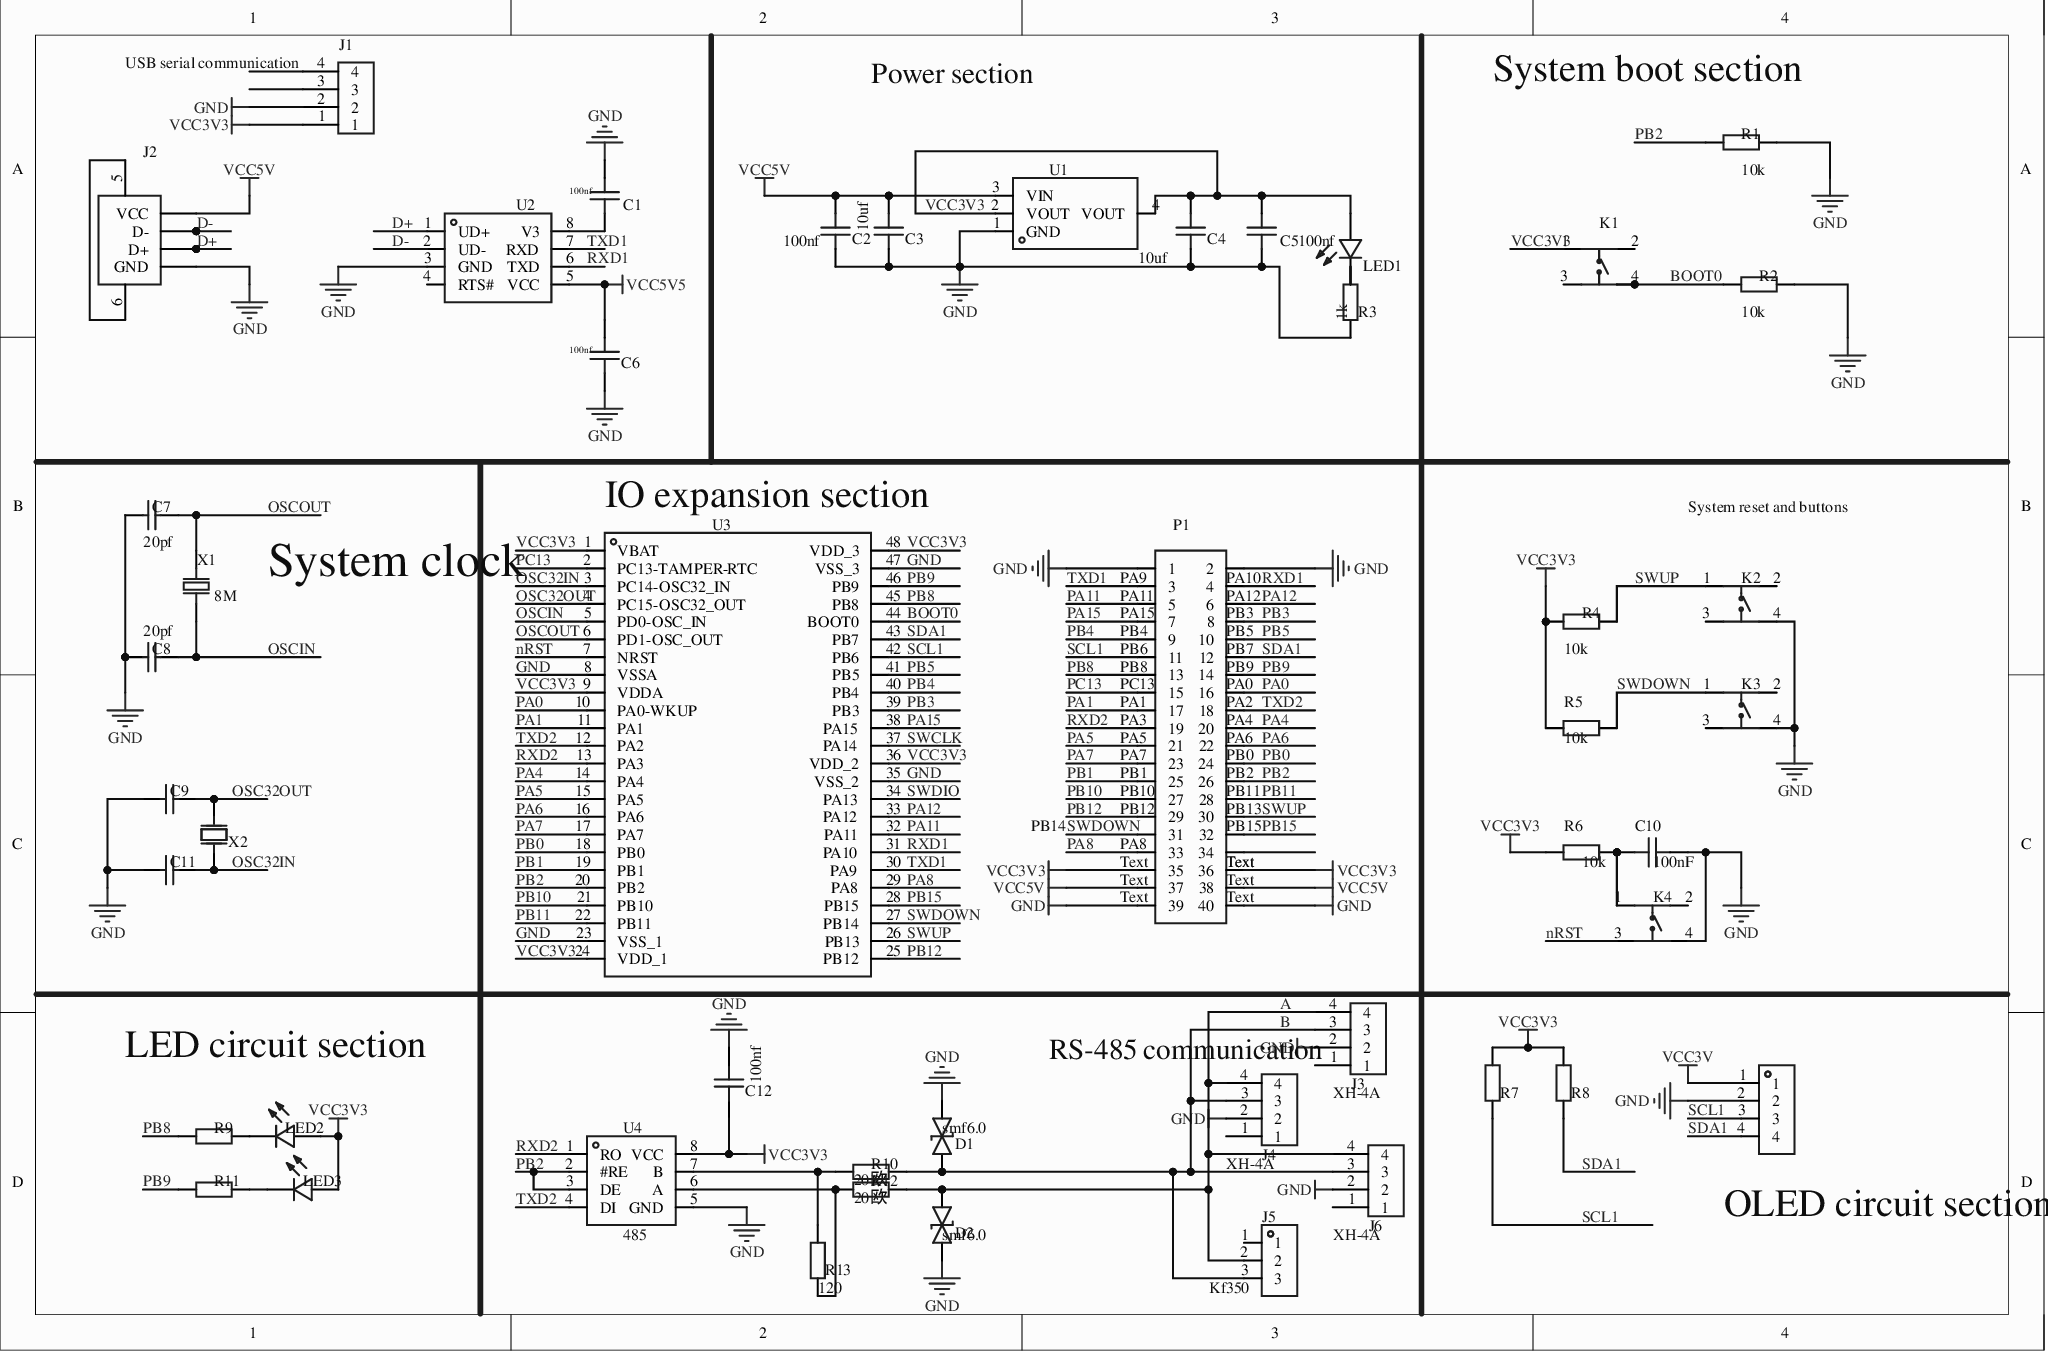
[diagram p0: MISC51869-3.schdoc]
# Altium project MISC51869-2.PrjPcb
1 sheet, 48 parts. Net scope: global (net labels, ports and power ports of the same name join across sheets).
Board file: MISC51869.pcbdoc

## Sheet MISC51869-3.schdoc
size 292 x 193 mm; SheetNumber: 1; SheetTotal: 1; Name: MISC51869

### Parts
C1  CC0603KRX7R9BB104  [C0603 - duplicate]  (value not drawn)
C2  CL21A106KAYNNNE  [C0805]  (value not drawn)
C3  CC0603KRX7R9BB104  [C0603 - duplicate]  (value not drawn)
C4  CL21A106KAYNNNE  [C0805]  (value not drawn)
C5  CC0603KRX7R9BB104  [C0603 - duplicate]  (value not drawn)
C6  CC0603KRX7R9BB104  [C0603 - duplicate]  (value not drawn)
C7  CL10C200JB8NNNC  [C0603c20pf]  (value not drawn)
C8  CL10C200JB8NNNC  [C0603c20pf]  (value not drawn)
C9  CL10C200JB8NNNC  [C0603c20pf]  (value not drawn)
C10  CL21A106KAYNNNE  [C0805]  (value not drawn)
C11  CL10C200JB8NNNC  [C0603c20pf]  (value not drawn)
C12  CC0603KRX7R9BB104  [C0603 - duplicate]  (value not drawn)
D1  SMF6.0CA_C2990473  [瞬态二极管]  (value not drawn)
D2  SMF6.0CA_C2990473  [瞬态二极管]  (value not drawn)
H1  PM254V-11-04-H85  [排母4p]  (value not drawn)
J1  XH-4A  [XH-4A]  (value not drawn)
J2  USB-B-Female-90  [USB-B_TH_USB-B-FEMALE-90]  (value not drawn)
J3  XH-4A  [XH-4A]  (value not drawn)
J4  XH-4A  [XH-4A]  (value not drawn)
J5  KF350-3.5-3P  [KF350-3.5-3P]  (value not drawn)
J6  XH-4A  [XH-4A]  (value not drawn)
K1  KH-6X6X5H-STM  [按键]  (value not drawn)
K2  KH-6X6X5H-STM  [复位按键]  (value not drawn)
K3  KH-6X6X5H-STM  [复位按键]  (value not drawn)
K4  KH-6X6X5H-STM  [复位按键]  (value not drawn)
LED1  FC-D1608HGK-572C  [LED0603-RD]  (value not drawn)
LED2  FC-D1608HGK-572C  [LED0603-RD]  (value not drawn)
LED3  FC-D1608HGK-572C  [LED0603-RD]  (value not drawn)
P1  Header-Male-2.54_2x20  [HDR-TH_40P-P2.54-V-M-R2-C20-S2.54]  (value not drawn)
R1  0603WAF1002T5E  [电阻R0603]  (value not drawn)
R2  0603WAF1002T5E  [电阻R0603]  (value not drawn)
R3  0603WAF1001T5E  [C0603 - duplicate]  (value not drawn)
R4  0603WAF1002T5E  [电阻R0603]  (value not drawn)
R5  0603WAF1002T5E  [电阻R0603]  (value not drawn)
R6  0603WAF1002T5E  [电阻R0603]  (value not drawn)
R7  0603WAF4701T5E  [R06034.7k]  (value not drawn)
R8  0603WAF4701T5E  [R06034.7k]  (value not drawn)
R9  0603WAF1001T5E  [R06031k]  (value not drawn)
R10  0805W8F200JT5E  [R0805]  (value not drawn)
R11  0603WAF1001T5E  [R06031k]  (value not drawn)
R12  0805W8F200JT5E  [R0805]  (value not drawn)
R13  0603WAF1200T5E  [R0603 - duplicate]  (value not drawn)
U1  AMS1117-3.3  [SOT-223-3_L6.5-W3.4-P2.30-LS7.0-BR]  (value not drawn)
U2  CH340N_C2977777  [SOP-8_L4.9-W3.9-P1.27-LS6.0-BL]  (value not drawn)
U3  STM32F103C8T6  [LQFP-48_L7.0-W7.0-P0.50-LS9.0-BL]  (value not drawn)
U4  SP3485EEN  [485SOP-8_L5.0-W4.0-P1.27-LS6.0-BL]  (value not drawn)
X1  Q13FC1350000400  [CRYSTAL-SMD_L5.0-W3.2]  (value not drawn)
X2  X50328MSB2GI  [FC-135R_L3.2-W1.5]  (value not drawn)

### Nets
GND: C1.2 C2.1 C3.2 C4.1 C5.1 C6.1 C7.1 C8.1 C9.1 C10.1 C11.1 C12.2 D1.2 D2.1 H1.2 J1.2 J2.4(GND) J3.2 J4.2 J6.2 K2.4 K3.4 K4.4 P1.1 P1.2 P1.39 P1.40 R1.2 R2.2 R3.1 U1.1(GND) U2.3(GND) U3.8(VSSA) U3.23(VSS_1) U3.35(VSS_2) U3.47(VSS_3) U4.5(GND)
VCC3V: H1.1
VCC3V3: C4.2 C5.2 C12.1 J1.1 K1.1 LED1.2(+) LED2.2(+) LED3.2(+) P1.35 P1.36 R4.1 R5.1 R6.1 R7.2 R8.2 U1.2(VOUT) U1.4(VOUT) U3.1(VBAT) U3.9(VDDA) U3.24(VDD_1) U3.36(VDD_2) U3.48(VDD_3) U4.8(VCC)
VCC5V: C2.2 C3.1 J2.1(VCC) P1.37 P1.38 U1.3(VIN)
VCC5V5: C6.2 U2.5(VCC)
A: D2.2 J3.4 J4.4 J5.2 J6.4 R12.2
B: D1.1 J3.3 J4.3 J5.3 J6.3 R10.2
BOOT0: K1.4 R2.1 U3.44(BOOT0)
D+: J2.3(D+) U2.1(UD+)
D-: J2.2(D-) U2.2(UD-)
nRST: K4.3 U3.7(NRST)
OSC32IN: C11.2 U3.3(PC14-OSC32_IN) X2.2(OSC2)
OSC32OUT: C9.2 U3.4(PC15-OSC32_OUT) X2.1(OSC1)
OSCIN: C8.2 U3.5(PD0-OSC_IN) X1.2
OSCOUT: C7.2 U3.6(PD1-OSC_OUT) X1.1
PA0: P1.16 U3.10(PA0-WKUP)
PA1: P1.17 U3.11(PA1)
PA4: P1.20 U3.14(PA4)
PA5: P1.21 U3.15(PA5)
PA6: P1.22 U3.16(PA6)
PA7: P1.23 U3.17(PA7)
PA8: P1.33 U3.29(PA8)
PA11: P1.5 U3.32(PA11)
PA12: P1.6 U3.33(PA12)
PA15: P1.7 U3.38(PA15)
PB0: P1.24 U3.18(PB0)
PB1: P1.25 U3.19(PB1)
PB2: P1.26 R1.1 U3.20(PB2) U4.2(#RE) U4.3(DE)
PB3: P1.8 U3.39(PB3)
PB4: P1.9 U3.40(PB4)
PB5: P1.10 U3.41(PB5)
PB8: P1.13 R9.1 U3.45(PB8)
PB9: P1.14 R11.1 U3.46(PB9)
PB10: P1.27 U3.21(PB10)
PB11: P1.28 U3.22(PB11)
PB12: P1.29 U3.25(PB12)
PB15: P1.32 U3.28(PB15)
PC13: P1.15 U3.2(PC13-TAMPER-RTC)
RXD1: P1.4 U2.6(TXD) U3.31(PA10)
RXD2: P1.19 U3.13(PA3) U4.1(RO)
SCL1: H1.3 P1.11 R7.1 U3.42(PB6)
SDA1: H1.4 P1.12 R8.1 U3.43(PB7)
SWCLK: U3.37(PA14)
SWDIO: U3.34(PA13)
SWDOWN: K3.1 P1.31 R5.2 U3.27(PB14)
SWUP: K2.1 P1.30 R4.2 U3.26(PB13)
TXD1: P1.3 U2.7(RXD) U3.30(PA9)
TXD2: P1.18 U3.12(PA2) U4.4(DI)
NetC1_1: C1.1 U2.8(V3)
NetC10_2: C10.2 K4.1 R6.2
NetJ2_5: J2.5(SH1) J2.6(SH2)
NetLED1_1: LED1.1(-) R3.2
NetLED2_1: LED2.1(-) R9.2
NetLED3_1: LED3.1(-) R11.2
NetR10_1: R10.1 R13.2 U4.7(B)
NetR12_1: R12.1 R13.1 U4.6(A)

Not connected (* = marked no-connect by the designer): J1 3* 4*; J3 1; J4 1; J5 1; J6 1; K1 2 3; K2 2 3; K3 2 3; K4 2; P1 34; U2 4(RTS#)

### Notes on the sheet
- (near J1) USB serial communication
- Power section
- (near R1) System boot section
- (near C1) 100nf
- 10uf
- (near R1) 10k
- (near C2) 100nf
- (near LED1) 100nf
- (near R3) 1k
- (near R2) 10k
- (near C6) 100nf
- 20pf
- System clock
- (near U3) IO expansion section
- (near P1) PA9
- (near P1) PA10
- System reset and buttons
- (near X1) 8M
- (near P1) PA11
- (near P1) PA15
- (near P1) PB4
- (near P1) PB6
- (near P1) PB8
- (near P1) PA12
- (near P1) PB3
- (near P1) PB5
- (near P1) PB7
- (near P1) PB9
- (near R4) 10k
- (near P1) PC13
- (near P1) PA1
- (near P1) PA3
- (near P1) PA5
- (near P1) PA7
- (near P1) PA0
- (near P1) PA2
- (near P1) PA4
- (near P1) PA6
- (near P1) PB0
- (near R5) 10k
- PB14
- (near P1) PB1
- (near P1) PB10
- (near P1) PB12
- (near P1) PA8
- (near P1) PB2
- (near P1) PB11
- (near P1) PB13
- (near P1) PB15
- (near P1) Text
- (near R6) 10k
- (near C10) 100nF
- LED circuit section
- (near C12) 100nf
- RS-485 communication
- (near J3) XH-4A
- (near R12) 20欧
- 20欧
- (near D1) smf6.0
- (near J4) XH-4A
- (near U4) 485
- (near R13) 120
- (near D2) smf6.0
- (near J5) Kf350
- (near J6) XH-4A
- (near H1) OLED circuit section

### Library data of the parts
C1 = CC0603KRX7R9BB104: OriginFootprint 2: C0603; UniqueId: 5fb4f22ffcb6a001; AddInBom: yes; Device: CC0603KRX7R9BB104; DesignItemID: CC0603KRX7R9BB104; SymbolName: CC0603KRX7R9BB104; FootprintName: C0603 - duplicate
C2 = CL21A106KAYNNNE: UniqueId: 21d50210554cb61f; AddInBom: yes; Device: CL21A106KAYNNNE; DesignItemID: CL21A106KAYNNNE; SymbolName: CL21A106KAYNNNE; FootprintName: C0805
C3 = CC0603KRX7R9BB104: OriginFootprint 2: C0603; UniqueId: ec64484c8c07847f; AddInBom: yes; Device: CC0603KRX7R9BB104; DesignItemID: CC0603KRX7R9BB104; SymbolName: CC0603KRX7R9BB104; FootprintName: C0603 - duplicate
C4 = CL21A106KAYNNNE: UniqueId: 623e2bb2442f04df; AddInBom: yes; Device: CL21A106KAYNNNE; DesignItemID: CL21A106KAYNNNE; SymbolName: CL21A106KAYNNNE; FootprintName: C0805
C5 = CC0603KRX7R9BB104: OriginFootprint 2: C0603; UniqueId: 05d417a4d81547fc; AddInBom: yes; Device: CC0603KRX7R9BB104; DesignItemID: CC0603KRX7R9BB104; SymbolName: CC0603KRX7R9BB104; FootprintName: C0603 - duplicate
C6 = CC0603KRX7R9BB104: OriginFootprint 2: C0603; UniqueId: d45ffe04e43665a4; AddInBom: yes; Device: CC0603KRX7R9BB104; DesignItemID: CC0603KRX7R9BB104; SymbolName: CC0603KRX7R9BB104; FootprintName: C0603 - duplicate
C7 = CL10C200JB8NNNC: UniqueId: 3007ca2539a35480; AddInBom: yes; Device: CL10C200JB8NNNC; DesignItemID: CL10C200JB8NNNC; SymbolName: CL10C200JB8NNNC; FootprintName: C0603c20pf
C8 = CL10C200JB8NNNC: UniqueId: 878ab3ab0cce2757; AddInBom: yes; Device: CL10C200JB8NNNC; DesignItemID: CL10C200JB8NNNC; SymbolName: CL10C200JB8NNNC; FootprintName: C0603c20pf
C9 = CL10C200JB8NNNC: UniqueId: 60e6893b044e2f17; AddInBom: yes; Device: CL10C200JB8NNNC; DesignItemID: CL10C200JB8NNNC; SymbolName: CL10C200JB8NNNC; FootprintName: C0603c20pf
C10 = CL21A106KAYNNNE: UniqueId: c1764753ee6525b4; AddInBom: yes; Device: CL21A106KAYNNNE; DesignItemID: CL21A106KAYNNNE; SymbolName: CL21A106KAYNNNE; FootprintName: C0805
C11 = CL10C200JB8NNNC: UniqueId: b49c3108c5288e9f; AddInBom: yes; Device: CL10C200JB8NNNC; DesignItemID: CL10C200JB8NNNC; SymbolName: CL10C200JB8NNNC; FootprintName: C0603c20pf
C12 = CC0603KRX7R9BB104: UniqueId: 4eba2014d94c20ef; OriginFootprint 2: C0603; AddInBom: yes; Device: CC0603KRX7R9BB104; DesignItemID: CC0603KRX7R9BB104; SymbolName: CC0603KRX7R9BB104; FootprintName: C0603 - duplicate
D1 = SMF6.0CA_C2990473: UniqueId: 07a0d5848cd81316; AddInBom: yes; Device: SMF6.0CA_C2990473; DesignItemID: SMF6.0CA_C2990473; SymbolName: SMF6.0CA_C2990473; FootprintName: TVS diode
D2 = SMF6.0CA_C2990473: UniqueId: fa5cd661465da5bc; AddInBom: yes; Device: SMF6.0CA_C2990473; DesignItemID: SMF6.0CA_C2990473; SymbolName: SMF6.0CA_C2990473; FootprintName: TVS diode
H1 = PM254V-11-04-H85: UniqueId: f372d9fd695b79ed; AddInBom: yes; Device: PM254V-11-04-H85; DesignItemID: PM254V-11-04-H85; SymbolName: PM254V-11-04-H85; FootprintName: Header 4P
J1 = XH-4A_1: OriginFootprint 2: CONN-TH_4P-P2.50_XH-4A; UniqueId: 9f49826860c2c79d; AddInBom: yes; Device: XH-4A_1; DesignItemID: XH-4A; SymbolName: XH-4A; FootprintName: XH-4A
J2 = USB-B-Female-90: UniqueId: 42913bc3a3449998; AddInBom: yes; ModelId: 427257db465a432d8a34b597c871403b; Device: USB-B-Female-90; DesignItemID: USB-B-Female-90; SymbolName: USB-B-Female-90; FootprintName: USB-B_TH_USB-B-FEMALE-90; ModelName: USB-B_TH_USB-B-FEMALE-90
J3 = XH-4A_1: UniqueId: 6ca7fcf0d18ad80e; OriginFootprint 2: CONN-TH_4P-P2.50_XH-4A; AddInBom: yes; Device: XH-4A_1; DesignItemID: XH-4A; SymbolName: XH-4A; FootprintName: XH-4A
J4 = XH-4A_1: UniqueId: 048fde32f53a6793; OriginFootprint 2: CONN-TH_4P-P2.50_XH-4A; AddInBom: yes; Device: XH-4A_1; DesignItemID: XH-4A; SymbolName: XH-4A; FootprintName: XH-4A
J5 = KF350-3.5-3P_1: UniqueId: c38aec87e6867e62; AddInBom: yes; Device: KF350-3.5-3P_1; DesignItemID: KF350-3.5-3P; SymbolName: KF350-3.5-3P; FootprintName: KF350-3.5-3P
J6 = XH-4A_1: UniqueId: ac8b08765cb6a234; OriginFootprint 2: CONN-TH_4P-P2.50_XH-4A; AddInBom: yes; Device: XH-4A_1; DesignItemID: XH-4A; SymbolName: XH-4A; FootprintName: XH-4A
K1 = KH-6X6X5H-STM: UniqueId: 28855386baaab8ba; AddInBom: yes; Device: KH-6X6X5H-STM; DesignItemID: KH-6X6X5H-STM; SymbolName: KH-6X6X5H-STM; FootprintName: Button
K2 = KH-6X6X5H-STM_1: UniqueId: e2dee5ee6a5fdee0; AddInBom: yes; Device: KH-6X6X5H-STM_1; DesignItemID: KH-6X6X5H-STM; SymbolName: KH-6X6X5H-STM; FootprintName: Reset button
K3 = KH-6X6X5H-STM_1: UniqueId: 177bbada0502c5f7; AddInBom: yes; Device: KH-6X6X5H-STM_1; DesignItemID: KH-6X6X5H-STM; SymbolName: KH-6X6X5H-STM; FootprintName: Reset button
K4 = KH-6X6X5H-STM_1: UniqueId: 787baf109c0c5026; AddInBom: yes; Device: KH-6X6X5H-STM_1; DesignItemID: KH-6X6X5H-STM; SymbolName: KH-6X6X5H-STM; FootprintName: Reset button
LED1 = FC-D1608HGK-572C: UniqueId: a4c4b307afb8d999; AddInBom: yes; ModelId: 1f0d29a91be547639d425604e9b96ebb; Device: FC-D1608HGK-572C; OriginFootprint 2: LED0603-RD; OriginFootprint 3: LED0603-RD; DesignItemID: FC-D1608HGK-572C; SymbolName: FC-D1608HGK-572C; FootprintName: LED0603-RD; ModelName: LED0603-RD
LED2 = FC-D1608HGK-572C: UniqueId: a245eb2d2aad9559; AddInBom: yes; ModelId: 1f0d29a91be547639d425604e9b96ebb; Device: FC-D1608HGK-572C; DesignItemID: FC-D1608HGK-572C; SymbolName: FC-D1608HGK-572C; FootprintName: LED0603-RD; OriginFootprint 2: LED0603-RD; OriginFootprint 3: LED0603-RD; ModelName: LED0603-RD
LED3 = FC-D1608HGK-572C: UniqueId: 01e448f2d6732d04; AddInBom: yes; ModelId: 1f0d29a91be547639d425604e9b96ebb; Device: FC-D1608HGK-572C; DesignItemID: FC-D1608HGK-572C; SymbolName: FC-D1608HGK-572C; FootprintName: LED0603-RD; OriginFootprint 2: LED0603-RD; OriginFootprint 3: LED0603-RD; ModelName: LED0603-RD
P1 = Header-Male-2.54_2x20: UniqueId: f88e3064cb77b82c; AddInBom: yes; Device: Header-Male-2.54_2x20; DesignItemID: Header-Male-2.54_2x20; SymbolName: Header-Male-2.54_2x20; FootprintName: HDR-TH_40P-P2.54-V-M-R2-C20-S2.54
R1 = 0603WAF1002T5E: UniqueId: 4e166b190d4de1c3; AddInBom: yes; Device: 0603WAF1002T5E; DesignItemID: 0603WAF1002T5E; SymbolName: 0603WAF1002T5E; FootprintName: Resistor R0603
R2 = 0603WAF1002T5E: UniqueId: 06442d24ab060343; AddInBom: yes; Device: 0603WAF1002T5E; DesignItemID: 0603WAF1002T5E; SymbolName: 0603WAF1002T5E; FootprintName: Resistor R0603
R3 = 0603WAF1001T5E: OriginFootprint 2: R0603; UniqueId: 6e26aea592918673; AddInBom: yes; Device: 0603WAF1001T5E; DesignItemID: 0603WAF1001T5E; SymbolName: 0603WAF1001T5E; FootprintName: C0603 - duplicate
R4 = 0603WAF1002T5E: UniqueId: 49359f7360e76581; AddInBom: yes; Device: 0603WAF1002T5E; DesignItemID: 0603WAF1002T5E; SymbolName: 0603WAF1002T5E; FootprintName: Resistor R0603
R5 = 0603WAF1002T5E: UniqueId: 96bd3269827a783e; AddInBom: yes; Device: 0603WAF1002T5E; DesignItemID: 0603WAF1002T5E; SymbolName: 0603WAF1002T5E; FootprintName: Resistor R0603
R6 = 0603WAF1002T5E: UniqueId: c9a24d22ca7022dc; AddInBom: yes; Device: 0603WAF1002T5E; DesignItemID: 0603WAF1002T5E; SymbolName: 0603WAF1002T5E; FootprintName: Resistor R0603
R7 = 0603WAF4701T5E: UniqueId: 01f5c70ff2630ee7; AddInBom: yes; Device: 0603WAF4701T5E; DesignItemID: 0603WAF4701T5E; SymbolName: 0603WAF4701T5E; FootprintName: R06034.7k
R8 = 0603WAF4701T5E: UniqueId: f0665cc51e401020; AddInBom: yes; Device: 0603WAF4701T5E; DesignItemID: 0603WAF4701T5E; SymbolName: 0603WAF4701T5E; FootprintName: R06034.7k
R9 = 0603WAF1001T5E_1: UniqueId: 7a9d276dcc23a651; AddInBom: yes; Device: 0603WAF1001T5E_1; DesignItemID: 0603WAF1001T5E; SymbolName: 0603WAF1001T5E; FootprintName: R06031k
R10 = 0805W8F200JT5E: UniqueId: 7663007c1f2bc029; AddInBom: yes; ModelId: 1f8f9bfd8e2b427398b06535d781678a; Device: 0805W8F200JT5E; DesignItemID: 0805W8F200JT5E; SymbolName: 0805W8F200JT5E; FootprintName: R0805; ModelName: R0805
R11 = 0603WAF1001T5E_1: UniqueId: 069ba0dc55a84bc8; AddInBom: yes; Device: 0603WAF1001T5E_1; DesignItemID: 0603WAF1001T5E; SymbolName: 0603WAF1001T5E; FootprintName: R06031k
R12 = 0805W8F200JT5E: UniqueId: f574a6082c36e6cb; AddInBom: yes; ModelId: 1f8f9bfd8e2b427398b06535d781678a; Device: 0805W8F200JT5E; DesignItemID: 0805W8F200JT5E; SymbolName: 0805W8F200JT5E; FootprintName: R0805; ModelName: R0805
R13 = 0603WAF1200T5E: UniqueId: ff7631ddbc1e2fda; AddInBom: yes; Device: 0603WAF1200T5E; DesignItemID: 0603WAF1200T5E; SymbolName: 0603WAF1200T5E; FootprintName: R0603 - duplicate
U1 = AMS1117-3.3: UniqueId: 48a4a086d8c42a18; AddInBom: yes; Device: AMS1117-3.3; DesignItemID: AMS1117-3.3; SymbolName: AMS1117-3.3; FootprintName: SOT-223-3_L6.5-W3.4-P2.30-LS7.0-BR
U2 = CH340N_C2977777: UniqueId: d74c11912b695046; AddInBom: yes; Device: CH340N_C2977777; DesignItemID: CH340N_C2977777; SymbolName: CH340N_C2977777; FootprintName: SOP-8_L4.9-W3.9-P1.27-LS6.0-BL
U3 = STM32F103C8T6: UniqueId: eac3f191c372887e; AddInBom: yes; Device: STM32F103C8T6; DesignItemID: STM32F103C8T6; SymbolName: STM32F103C8T6; FootprintName: LQFP-48_L7.0-W7.0-P0.50-LS9.0-BL
U4 = SP3485EEN: UniqueId: e5d1bee62801ccc5; AddInBom: yes; Device: SP3485EEN; DesignItemID: SP3485EEN; SymbolName: SP3485EEN; FootprintName: 485SOP-8_L5.0-W4.0-P1.27-LS6.0-BL
X1 = Q13FC1350000400: UniqueId: 3fdc0bfeb28a4101; AddInBom: yes; ModelId: d7c39c66443246ff83c2003c1e1eb6f1; Device: Q13FC1350000400; DesignItemID: Q13FC1350000400; SymbolName: Q13FC1350000400; FootprintName: CRYSTAL-SMD_L5.0-W3.2; ModelName: CRYSTAL-SMD_L5.0-W3.2
X2 = X50328MSB2GI: UniqueId: 4e2fbb5f22124518; AddInBom: yes; ModelId: 751105e878f044059ef0ee72de95f96e; Device: X50328MSB2GI; DesignItemID: X50328MSB2GI; SymbolName: X50328MSB2GI; FootprintName: FC-135R_L3.2-W1.5; ModelName: FC-135R_L3.2-W1.5